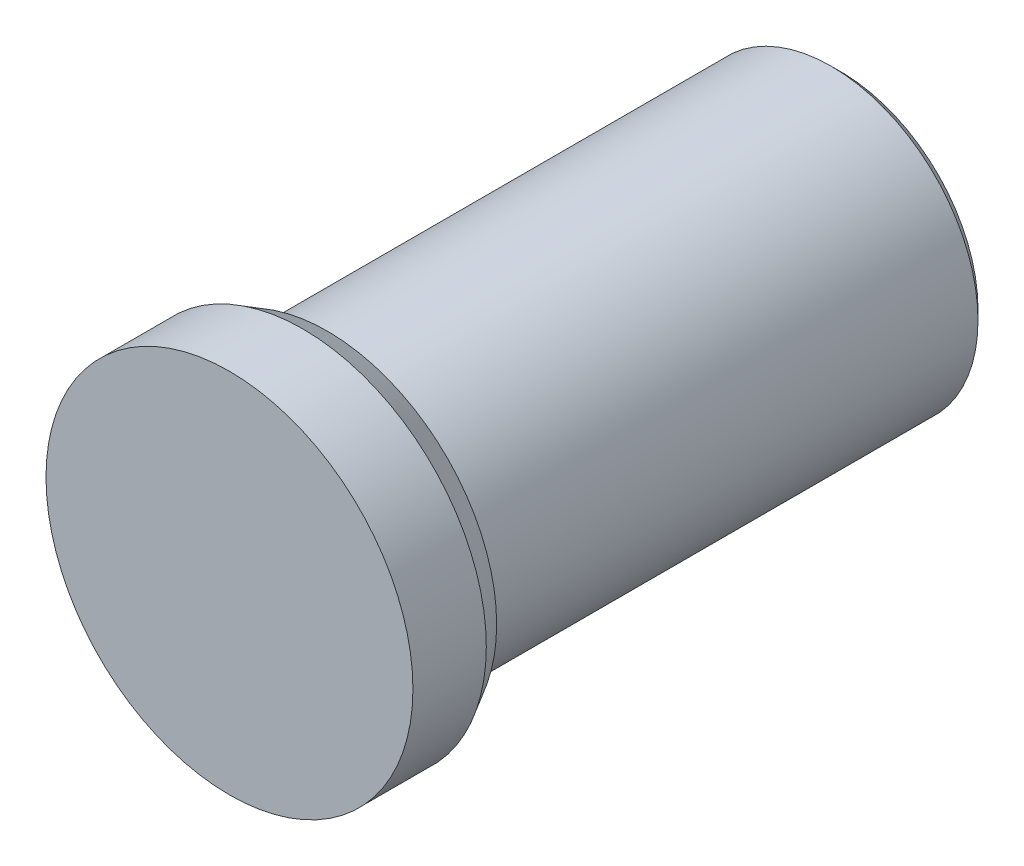
from build123d import *

# Parameters (mm, degrees)
SKETCH_1_R      = 30
EXTRUDE_1_DEPTH = 105
SKETCH_2_R      = 37.5
EXTRUDE_2_DEPTH = 20
CHAMFER_2_SIZE  = 2
SKETCH_3_W      = 1
SKETCH_3_H      = 2
CHAMFER_3_SIZE  = 5
CHAMFER_3_SIZE2 = 2.886751346


with BuildPart() as part:
    # 草图1 → 凸台-拉伸1 (new body)
    with BuildSketch(Plane.XY):
        Circle(SKETCH_1_R)
    extrude(amount=EXTRUDE_1_DEPTH)

    # 草图2 → 凸台-拉伸2 (add)
    with BuildSketch(Plane.XY.offset(105)):
        Circle(SKETCH_2_R)
    extrude(amount=EXTRUDE_2_DEPTH)

    # 倒角2
    chamfer_2_edges = [part.edges().sort_by_distance(p)[0] for p in [
        (-30, 0, 0),
    ]]
    chamfer(chamfer_2_edges, length=CHAMFER_2_SIZE)

    # 草图3 → 切除-旋转1 (revolve, cut)
    with BuildSketch(Plane(origin=(0, 0, 0), x_dir=(1, 0, 0), z_dir=(0, 1, 0))):
        with Locations((29.5, -104)):
            Rectangle(SKETCH_3_W, SKETCH_3_H)
    revolve(axis=Axis((0, 0, 105), (0, 0, -1)), mode=Mode.SUBTRACT)

    # 倒角3
    chamfer_3_edges = [part.edges().sort_by_distance(p)[0] for p in [
        (-37.5, 0, 105),
    ]]
    chamfer_3_side = [part.faces().sort_by_distance(p)[0] for p in [
        (-37.5, 0, 115),
    ]]
    chamfer(chamfer_3_edges, length=CHAMFER_3_SIZE, length2=CHAMFER_3_SIZE2, reference=chamfer_3_side[0])


solid = part.part
